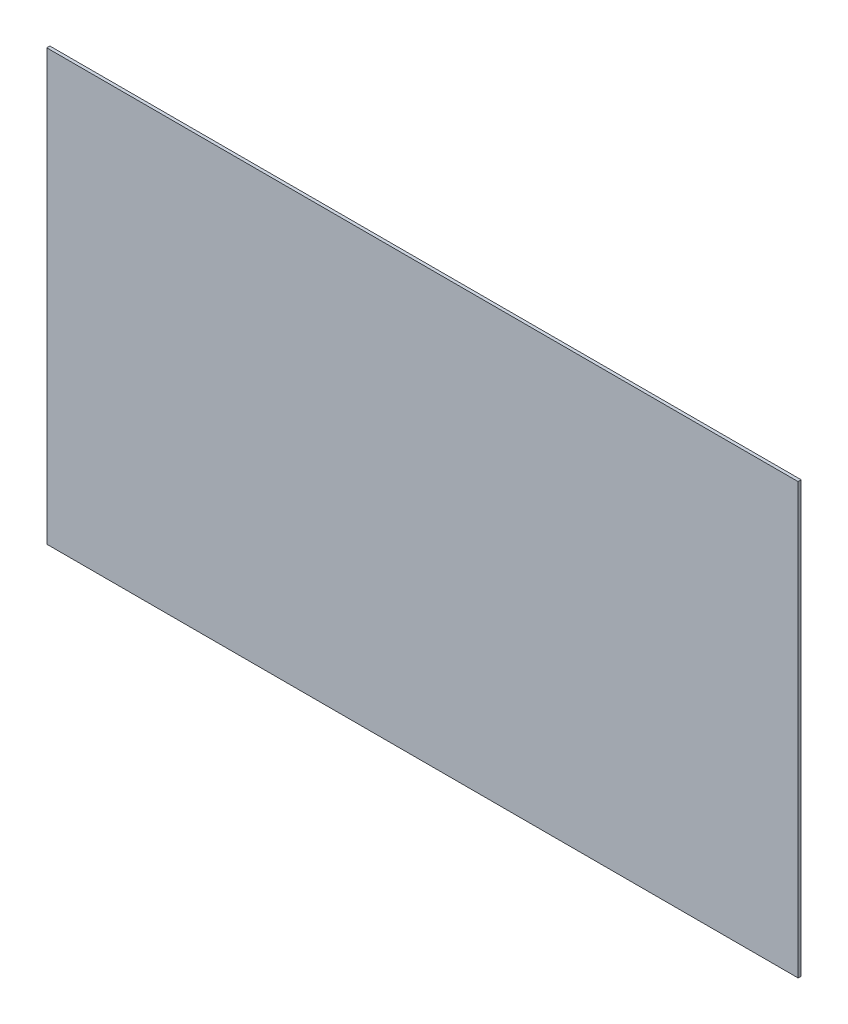
from build123d import *

# Parameters (mm, degrees)
SKETCH_1_W      = 1206
SKETCH_1_H      = 690
EXTRUDE_1_DEPTH = 5


with BuildPart() as part:
    # 草图1 → 凸台-拉伸1 (new body)
    with BuildSketch(Plane.XY):
        Rectangle(SKETCH_1_W, SKETCH_1_H)
    extrude(amount=EXTRUDE_1_DEPTH)


solid = part.part
